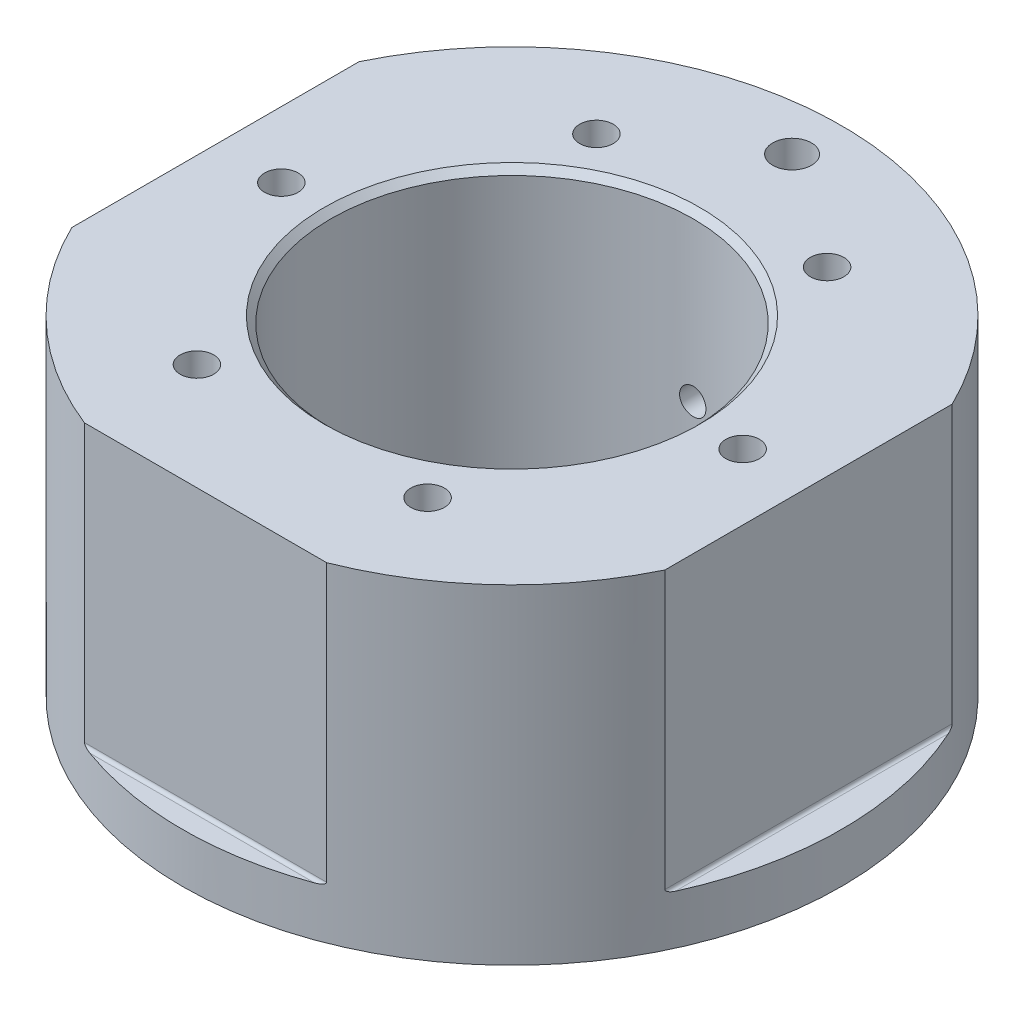
from build123d import *

# Parameters (mm, degrees)
SKETCH1_R                    = 100
BOSS_EXTRUDE1_DEPTH          = 100
CUT_EXTRUDE1_START           = -85
CUT_EXTRUDE1_DEPTH           = 85
SKETCH3_R                    = 55
CUT_EXTRUDE2_DEPTH           = 174.205080757
CHAMFER1_SIZE                = 2
SKETCH10_R                   = 4
CUT_EXTRUDE3_DEPTH           = 174.205080757
CIRPATTERN1_COUNT            = 6
G1_4_TAPPED_HOLE1_D          = 11.8
G1_4_TAPPED_HOLE1_DEPTH      = 10
G1_4_TAPPED_HOLE1_TIP        = 3.545077652
F_8_0_8_DIAMETER_HOLE1_D     = 8
F_8_0_8_DIAMETER_HOLE1_DEPTH = 60
F_8_0_8_DIAMETER_HOLE1_TIP   = 2.403442476
F_8_0_8_DIAMETER_HOLE2_D     = 8
F_8_0_8_DIAMETER_HOLE2_DEPTH = 60
F_8_0_8_DIAMETER_HOLE2_TIP   = 2.403442476
FILLET1_R                    = 1


with BuildPart() as part:
    # Sketch1 → Boss-Extrude1 (new body)
    with BuildSketch(Plane(origin=(0, 0, 0), x_dir=(1, 0, 0), z_dir=(0, 1, 0))):
        with Locations(Location((0, 0, 0), (0, 0, 270))):
            Circle(SKETCH1_R)
    extrude(amount=BOSS_EXTRUDE1_DEPTH)

    # Sketch2 → Cut-Extrude1 (cut)
    with BuildSketch(Plane(origin=(0, 100, 0), x_dir=(1, 0, 0), z_dir=(0, 1, 0)).offset(CUT_EXTRUDE1_START)):
        with BuildLine():
            Line((-36.755951899, -93), (36.755951899, -93))
            ThreePointArc((36.755951899, -93), (0, -100), (-36.755951899, -93))
        make_face()
        with BuildLine():
            Line((-90, -43.588989435), (-90, 43.588989435))
            ThreePointArc((-90, 43.588989435), (-100, 0), (-90, -43.588989435))
        make_face()
        with BuildLine():
            Line((90, -43.588989435), (90, 43.588989435))
            ThreePointArc((90, 43.588989435), (100, 0), (90, -43.588989435))
        make_face()
    extrude(amount=CUT_EXTRUDE1_DEPTH, mode=Mode.SUBTRACT)

    # Sketch3 → Cut-Extrude2 (cut, through all)
    with BuildSketch(Plane(origin=(0, 100, 0), x_dir=(1, 0, 0), z_dir=(0, 1, 0))):
        with Locations(Location((0, 0, 0), (0, 0, 270))):
            Circle(SKETCH3_R)
    extrude(amount=-CUT_EXTRUDE2_DEPTH, mode=Mode.SUBTRACT)

    # Chamfer1
    chamfer1_edges = [part.edges().sort_by_distance(p)[0] for p in [
        (0, 0, -55),
        (0, 100, -55),
    ]]
    chamfer(chamfer1_edges, length=CHAMFER1_SIZE)

    # Sketch6 → M12 Tapped Hole1 (revolve, cut)
    with BuildSketch(Plane(origin=(-35, 100, -60.621778265), x_dir=(0, 0, 1), z_dir=(1, 0, 0))):
        Polygon((0, 0), (0, 38.314389157), (5.1, 35.25), (5.1, 0), align=None)
    m12_tapped_hole1 = revolve(axis=Axis((-35, 106.35, -60.621778265), (0, -1, 0)), mode=Mode.SUBTRACT)

    # Sketch9 → M12 Tapped Hole2 (revolve, cut)
    with BuildSketch(Plane(origin=(-35, 0, -60.621778265), x_dir=(0, 0, -1), z_dir=(1, 0, 0))):
        Polygon((0, 0), (0, 38.314389157), (5.1, 35.25), (5.1, 0), align=None)
    m12_tapped_hole2 = revolve(axis=Axis((-35, -6.35, -60.621778265), (0, 1, 0)), mode=Mode.SUBTRACT)

    # Sketch10 → Cut-Extrude3 (cut, through all)
    with BuildSketch(Plane.XZ):
        with Locations(Location((-35, -60.621778265, 0), (0, 0, 270))):
            Circle(SKETCH10_R)
    cut_extrude3 = extrude(amount=-CUT_EXTRUDE3_DEPTH, mode=Mode.SUBTRACT)

    # CirPattern1: M12 Tapped Hole1, M12 Tapped Hole2, Cut-Extrude3 ×6 about axis
    cirpattern1_axis = Axis((0, 0, 0), (0, 1, 0))
    add([m12_tapped_hole1.rotate(cirpattern1_axis, i * 360 / CIRPATTERN1_COUNT) for i in range(1, CIRPATTERN1_COUNT)], mode=Mode.SUBTRACT)
    add([m12_tapped_hole2.rotate(cirpattern1_axis, i * 360 / CIRPATTERN1_COUNT) for i in range(1, CIRPATTERN1_COUNT)], mode=Mode.SUBTRACT)
    add([cut_extrude3.rotate(cirpattern1_axis, i * 360 / CIRPATTERN1_COUNT) for i in range(1, CIRPATTERN1_COUNT)], mode=Mode.SUBTRACT)

    # G1/4 Tapped Hole1
    with Locations(Plane(origin=(0, 100, 0), x_dir=(1, 0, 0), z_dir=(0, 1, 0))):
        with Locations((0, 85)):
            Hole(G1_4_TAPPED_HOLE1_D / 2, depth=G1_4_TAPPED_HOLE1_DEPTH)
            with Locations((0, 0, -(G1_4_TAPPED_HOLE1_DEPTH + G1_4_TAPPED_HOLE1_TIP / 2))):  # 118° drill point
                Cone(0, G1_4_TAPPED_HOLE1_D / 2, G1_4_TAPPED_HOLE1_TIP, mode=Mode.SUBTRACT)

    # Ø8.0 (8) Diameter Hole1
    with Locations(Plane(origin=(0, 100, 0), x_dir=(1, 0, 0), z_dir=(0, 1, 0))):
        with Locations((0, 85)):
            Hole(F_8_0_8_DIAMETER_HOLE1_D / 2, depth=F_8_0_8_DIAMETER_HOLE1_DEPTH)
            with Locations((0, 0, -(F_8_0_8_DIAMETER_HOLE1_DEPTH + F_8_0_8_DIAMETER_HOLE1_TIP / 2))):  # 118° drill point
                Cone(0, F_8_0_8_DIAMETER_HOLE1_D / 2, F_8_0_8_DIAMETER_HOLE1_TIP, mode=Mode.SUBTRACT)

    # Ø8.0 (8) Diameter Hole2
    with Locations(Plane(origin=(0, 50, -100), x_dir=(-1, 0, 0), z_dir=(0, 0, -1))):
        with Locations((0, 0)):
            Hole(F_8_0_8_DIAMETER_HOLE2_D / 2, depth=F_8_0_8_DIAMETER_HOLE2_DEPTH)
            with Locations((0, 0, -(F_8_0_8_DIAMETER_HOLE2_DEPTH + F_8_0_8_DIAMETER_HOLE2_TIP / 2))):  # 118° drill point
                Cone(0, F_8_0_8_DIAMETER_HOLE2_D / 2, F_8_0_8_DIAMETER_HOLE2_TIP, mode=Mode.SUBTRACT)

    # Fillet1
    fillet1_edges = [part.edges().sort_by_distance(p)[0] for p in [
        (0, 15, 93),
        (-90, 15, 0),
        (90, 15, 0),
    ]]
    fillet(fillet1_edges, radius=FILLET1_R)


solid = part.part
